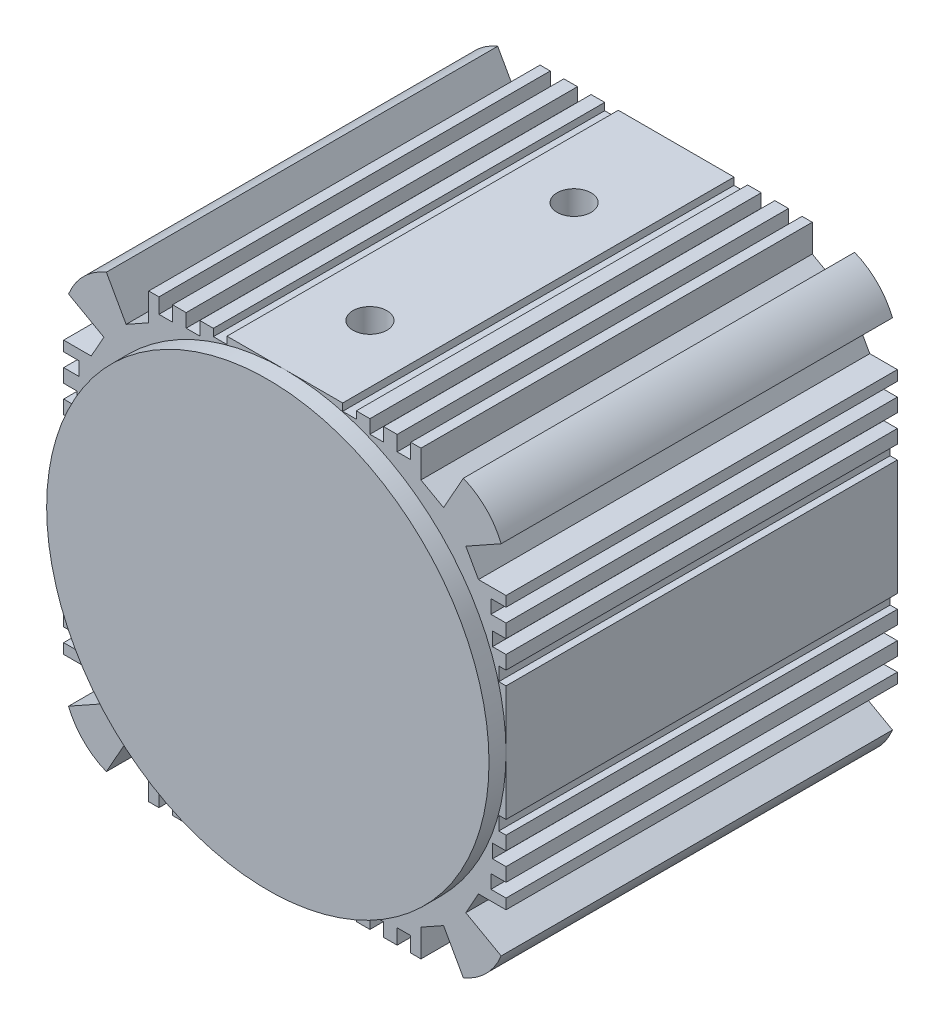
from build123d import *

# Parameters (mm, degrees)
SKETCH2_W                     = 130
SKETCH2_H                     = 130
BOSS_EXTRUDE2_DEPTH           = 120
SKETCH3_R                     = 110.525507452
SKETCH3_R_2                   = 65
CUT_EXTRUDE1_DEPTH            = 5
FILLET1_R                     = 20
SKETCH4_W                     = 4
SKETCH4_H                     = 15.569973817
SKETCH4_H_2                   = 23.441880492
SKETCH4_H_3                   = 22.368627222
CUT_EXTRUDE2_DEPTH            = 200
CIRPATTERN2_COUNT             = 4
CIRPATTERN2_COPY_1_SKETCH_W   = 4
CIRPATTERN2_COPY_1_SKETCH_H   = 15.569973817
CIRPATTERN2_COPY_1_SKETCH_H_2 = 23.441880492
CIRPATTERN2_COPY_1_SKETCH_H_3 = 22.368627222
CIRPATTERN2_COPY_1_DEPTH      = 200
CIRPATTERN2_COPY_2_SKETCH_W   = 4
CIRPATTERN2_COPY_2_SKETCH_H   = 15.569973817
CIRPATTERN2_COPY_2_SKETCH_H_2 = 23.441880492
CIRPATTERN2_COPY_2_SKETCH_H_3 = 22.368627222
CIRPATTERN2_COPY_2_DEPTH      = 200
CIRPATTERN2_COPY_3_SKETCH_W   = 4
CIRPATTERN2_COPY_3_SKETCH_H   = 15.569973817
CIRPATTERN2_COPY_3_SKETCH_H_2 = 23.441880492
CIRPATTERN2_COPY_3_SKETCH_H_3 = 22.368627222
CIRPATTERN2_COPY_3_DEPTH      = 200
SKETCH5_R                     = 5
CUT_EXTRUDE3_DEPTH            = 10


with BuildPart() as part:
    # Sketch2 → Boss-Extrude2 (new body)
    with BuildSketch(Plane.XY):
        Rectangle(SKETCH2_W, SKETCH2_H)
    extrude(amount=BOSS_EXTRUDE2_DEPTH)

    # Sketch3 → Cut-Extrude1 (cut)
    with BuildSketch(Plane.XY.offset(120)):
        Circle(SKETCH3_R)
        with Locations(Location((0, 0, 0), (0, 0, 180))):
            Circle(SKETCH3_R_2, mode=Mode.SUBTRACT)
    extrude(amount=-CUT_EXTRUDE1_DEPTH, mode=Mode.SUBTRACT)

    # Fillet1
    fillet1_edges = [part.edges().sort_by_distance(p)[0] for p in [
        (65, -65, 57.5),
        (-65, -65, 57.5),
        (-65, 65, 57.5),
        (65, 65, 57.5),
    ]]
    fillet(fillet1_edges, radius=FILLET1_R)

    # Sketch4 → Cut-Extrude2 (cut)
    with BuildSketch(Plane.XY.offset(115)):
        Polygon((-55.12283176, 68.343885556), (-46.644079041, 53.184903421), (-40, 56.901083224), (-40, 68.343885556), align=None)
        with Locations((-35, 68.343885556)):
            Rectangle(SKETCH4_W, SKETCH4_H)
        with Locations((-27, 72.752455261)):
            Rectangle(SKETCH4_W, SKETCH4_H_2)
        with Locations((-19, 74.056813123)):
            Rectangle(SKETCH4_W, SKETCH4_H_3)
    cut_extrude2 = extrude(amount=-CUT_EXTRUDE2_DEPTH, mode=Mode.SUBTRACT)

    # Mirror1: Cut-Extrude2 across plane
    add(cut_extrude2.mirror(Plane(origin=(0, 0, 0), x_dir=(0, 0, 1), z_dir=(1, 0, 0))), mode=Mode.SUBTRACT)

    # CirPattern2: Cut-Extrude2 ×4 about axis
    cirpattern2_axis = Axis((0, 0, 0), (0, 0, 1))
    for i in range(1, CIRPATTERN2_COUNT):
        add(cut_extrude2.rotate(cirpattern2_axis, i * 360 / CIRPATTERN2_COUNT), mode=Mode.SUBTRACT)

    # CirPattern2 copy 1 sketch → CirPattern2 copy 1 (cut)
    with BuildSketch(Plane(origin=(0, 0, 115), x_dir=(0, -1, 0), z_dir=(0, 0, 1))):
        Polygon((-55.12283176, -68.343885556), (-46.644079041, -53.184903421), (-40, -56.901083224), (-40, -68.343885556), align=None)
        with Locations((-35, -68.343885556)):
            Rectangle(CIRPATTERN2_COPY_1_SKETCH_W, CIRPATTERN2_COPY_1_SKETCH_H)
        with Locations((-27, -72.752455261)):
            Rectangle(CIRPATTERN2_COPY_1_SKETCH_W, CIRPATTERN2_COPY_1_SKETCH_H_2)
        with Locations((-19, -74.056813123)):
            Rectangle(CIRPATTERN2_COPY_1_SKETCH_W, CIRPATTERN2_COPY_1_SKETCH_H_3)
    extrude(amount=-CIRPATTERN2_COPY_1_DEPTH, mode=Mode.SUBTRACT)

    # CirPattern2 copy 2 sketch → CirPattern2 copy 2 (cut)
    with BuildSketch(Plane.XY.offset(115)):
        Polygon((-55.12283176, -68.343885556), (-46.644079041, -53.184903421), (-40, -56.901083224), (-40, -68.343885556), align=None)
        with Locations((-35, -68.343885556)):
            Rectangle(CIRPATTERN2_COPY_2_SKETCH_W, CIRPATTERN2_COPY_2_SKETCH_H)
        with Locations((-27, -72.752455261)):
            Rectangle(CIRPATTERN2_COPY_2_SKETCH_W, CIRPATTERN2_COPY_2_SKETCH_H_2)
        with Locations((-19, -74.056813123)):
            Rectangle(CIRPATTERN2_COPY_2_SKETCH_W, CIRPATTERN2_COPY_2_SKETCH_H_3)
    extrude(amount=-CIRPATTERN2_COPY_2_DEPTH, mode=Mode.SUBTRACT)

    # CirPattern2 copy 3 sketch → CirPattern2 copy 3 (cut)
    with BuildSketch(Plane(origin=(0, 0, 115), x_dir=(0, 1, 0), z_dir=(0, 0, 1))):
        Polygon((-55.12283176, -68.343885556), (-46.644079041, -53.184903421), (-40, -56.901083224), (-40, -68.343885556), align=None)
        with Locations((-35, -68.343885556)):
            Rectangle(CIRPATTERN2_COPY_3_SKETCH_W, CIRPATTERN2_COPY_3_SKETCH_H)
        with Locations((-27, -72.752455261)):
            Rectangle(CIRPATTERN2_COPY_3_SKETCH_W, CIRPATTERN2_COPY_3_SKETCH_H_2)
        with Locations((-19, -74.056813123)):
            Rectangle(CIRPATTERN2_COPY_3_SKETCH_W, CIRPATTERN2_COPY_3_SKETCH_H_3)
    extrude(amount=-CIRPATTERN2_COPY_3_DEPTH, mode=Mode.SUBTRACT)

    # Sketch5 → Cut-Extrude3 (cut)
    with BuildSketch(Plane(origin=(0, 65, 0), x_dir=(1, 0, 0), z_dir=(0, 1, 0))):
        with Locations(Location((0, -90, 0), (0, 0, 270))):
            Circle(SKETCH5_R)
        with Locations(Location((0, -30, 0), (0, 0, 270))):
            Circle(SKETCH5_R)
    extrude(amount=-CUT_EXTRUDE3_DEPTH, mode=Mode.SUBTRACT)


solid = part.part
